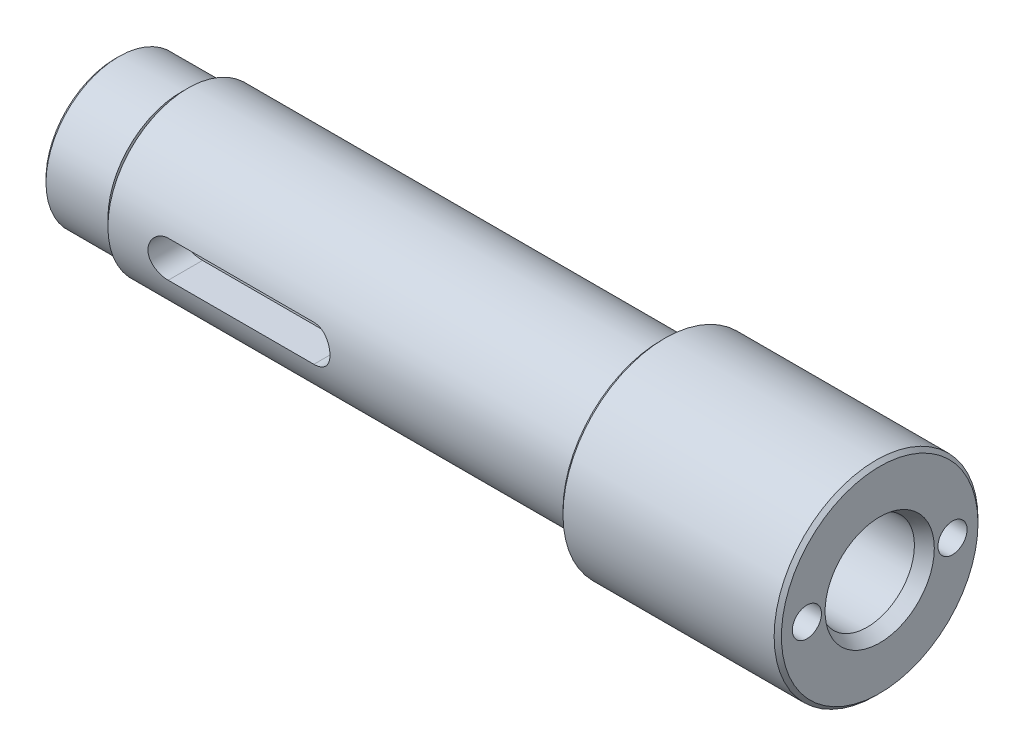
from build123d import *
from OCP.BRepFilletAPI import BRepFilletAPI_MakeChamfer

# Parameters (mm, degrees)
SKETCH_1_R                = 14
SKETCH_1_R_2              = 6.5
EXTRUDE_1_DEPTH           = 105
SKETCH_2_R                = 14
SKETCH_2_R_2              = 11
CUT_EXTRUDE_1_DEPTH       = 75
CUT_EXTRUDE_2_DEPTH       = 25
SKETCH_7_R                = 11
SKETCH_7_R_2              = 10
CUT_EXTRUDE_3_DEPTH       = 10
SKETCH_8_W                = 1
SKETCH_8_H                = 1.5
CHAMFER_1_SIZE            = 0.5
HOLE_WIZARD_4_0_4_1_D     = 4
HOLE_WIZARD_4_0_4_1_DEPTH = 8
HOLE_WIZARD_4_0_4_1_TIP   = 1.201721238
CHAMFER_2_SIZE            = 1
CHAMFER_2_SIZE2           = 1.732050808


with BuildPart() as part:
    # 草图1 → 凸台-拉伸1 (new body)
    with BuildSketch(Plane(origin=(0, 0, 0), x_dir=(0, 0, -1), z_dir=(1, 0, 0))):
        Circle(SKETCH_1_R)
        Circle(SKETCH_1_R_2, mode=Mode.SUBTRACT)
    extrude(amount=EXTRUDE_1_DEPTH)

    # 草图2 → 切除-拉伸1 (cut)
    with BuildSketch(Plane.ZY):
        Circle(SKETCH_2_R)
        Circle(SKETCH_2_R_2, mode=Mode.SUBTRACT)
    extrude(amount=-CUT_EXTRUDE_1_DEPTH, mode=Mode.SUBTRACT)

    # 草图4 → 切除-拉伸2 (cut, symmetric)
    with BuildSketch(Plane.XY):
        with BuildLine():
            Line((18, 2.5), (38, 2.5))
            ThreePointArc((38, 2.5), (40.5, 0), (38, -2.5))
            Line((38, -2.5), (18, -2.5))
            ThreePointArc((18, -2.5), (15.5, 0), (18, 2.5))
        make_face()
    extrude(amount=CUT_EXTRUDE_2_DEPTH, both=True, mode=Mode.SUBTRACT)

    # 草图7 → 切除-拉伸3 (cut)
    with BuildSketch(Plane.ZY):
        Circle(SKETCH_7_R)
        Circle(SKETCH_7_R_2, mode=Mode.SUBTRACT)
    extrude(amount=-CUT_EXTRUDE_3_DEPTH, mode=Mode.SUBTRACT)

    # 草图8 → 切除-旋转2 (revolve, cut)
    with BuildSketch(Plane.XY, mode=Mode.PRIVATE) as cut_revolve_2_sk:
        with Locations((9.5, 9.25)):
            Rectangle(SKETCH_8_W, SKETCH_8_H)
    revolve(cut_revolve_2_sk.sketch.rotate(Axis((0, 0, 0), (1, 0, 0)), 90), axis=Axis((0, 0, 0), (1, 0, 0)), mode=Mode.SUBTRACT)

    # 倒角1
    chamfer_1_edges = [part.edges().sort_by_distance(p)[0] for p in [
        (75, 0, 14),
        (105, 0, 14),
        (0, 0, -10),
    ]]
    chamfer(chamfer_1_edges, length=CHAMFER_1_SIZE)

    # Ø4.0 (4) 直径孔1
    with Locations(Plane(origin=(105, 0, 0), x_dir=(0, 0, -1), z_dir=(1, 0, 0))):
        with Locations((-10, 0), (10, 0)):
            Hole(HOLE_WIZARD_4_0_4_1_D / 2, depth=HOLE_WIZARD_4_0_4_1_DEPTH)
            with Locations((0, 0, -(HOLE_WIZARD_4_0_4_1_DEPTH + HOLE_WIZARD_4_0_4_1_TIP / 2))):  # 118° drill point
                Cone(0, HOLE_WIZARD_4_0_4_1_D / 2, HOLE_WIZARD_4_0_4_1_TIP, mode=Mode.SUBTRACT)

    # 倒角2: one chamfer whose edges measure the first distance from different faces: ONE call of the kernel's chamfer builder (chamfer() names one face for all edges)
    chamfer_2_edges_1 = [part.edges().sort_by_distance(p)[0] for p in [
        (0, 0, 6.5),
    ]]
    chamfer_2_side_1 = [part.faces().sort_by_distance(p)[0] for p in [
        (0, 0, -9.231299423),
    ]]
    chamfer_2_edges_2 = [part.edges().sort_by_distance(p)[0] for p in [
        (105, 0, 6.5),
    ]]
    chamfer_2_side_2 = [part.faces().sort_by_distance(p)[0] for p in [
        (105, 0, 13.118162338),
    ]]
    chamfer_2 = BRepFilletAPI_MakeChamfer(part.part.solid().wrapped)
    for e in chamfer_2_edges_1:
        chamfer_2.Add(CHAMFER_2_SIZE, CHAMFER_2_SIZE2, e.wrapped, chamfer_2_side_1[0].wrapped)  # the first distance lies on this face
    for e in chamfer_2_edges_2:
        chamfer_2.Add(CHAMFER_2_SIZE, CHAMFER_2_SIZE2, e.wrapped, chamfer_2_side_2[0].wrapped)  # the first distance lies on this face
    add(Compound.cast(chamfer_2.Shape()), mode=Mode.REPLACE)


solid = part.part
